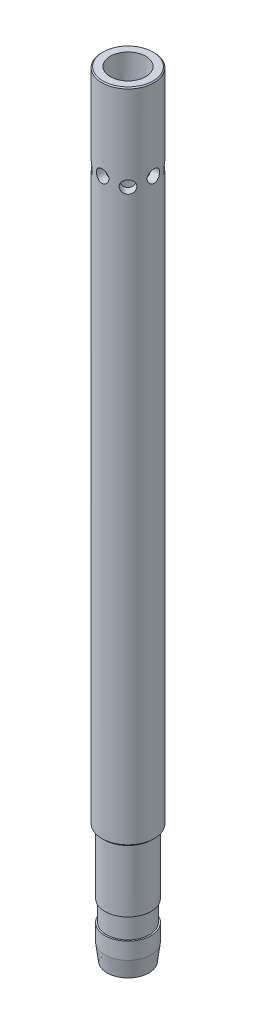
from build123d import *

# Parameters (mm, degrees)
SKETCH1_R           = 12.5
SKETCH1_R_2         = 8.5
BOSS_EXTRUDE1_DEPTH = 371
SKETCH2_R           = 16
SKETCH2_R_2         = 11
CUT_EXTRUDE1_DEPTH  = 56
SKETCH3_W           = 0.7
SKETCH3_H           = 10
CHAMFER1_SIZE       = 8
CHAMFER1_SIZE2      = 1
CHAMFER2_SIZE       = 1
SKETCH7_R           = 3
CUT_EXTRUDE4_DEPTH  = 24
CIRPATTERN2_COUNT   = 4
CHAMFER3_SIZE       = 0.5
SKETCH9_R           = 3
CUT_EXTRUDE11_DEPTH = 372.420920358
CIRPATTERN3_COUNT   = 4


with BuildPart() as part:
    # Sketch1 → Boss-Extrude1 (new body)
    with BuildSketch(Plane(origin=(0, 0, 0), x_dir=(1, 0, 0), z_dir=(0, 1, 0))):
        with Locations(Location((0, 0, 0), (0, 0, 270))):
            Circle(SKETCH1_R)
        with Locations(Location((0, 0, 0), (0, 0, 270))):
            Circle(SKETCH1_R_2, mode=Mode.SUBTRACT)
    extrude(amount=BOSS_EXTRUDE1_DEPTH)

    # Sketch2 → Cut-Extrude1 (cut)
    with BuildSketch(Plane.XZ):
        Circle(SKETCH2_R)
        with Locations(Location((0, 0, 0), (0, 0, 270))):
            Circle(SKETCH2_R_2, mode=Mode.SUBTRACT)
    extrude(amount=-CUT_EXTRUDE1_DEPTH, mode=Mode.SUBTRACT)

    # Sketch3 → Cut-Revolve1 (revolve, cut)
    with BuildSketch(Plane.XY, mode=Mode.PRIVATE) as cut_revolve1_sk:
        with Locations((10.65, 21)):
            Rectangle(SKETCH3_W, SKETCH3_H)
    revolve(cut_revolve1_sk.sketch.rotate(Axis((0, 357.5, 0), (0, -1, 0)), 270), axis=Axis((0, 357.5, 0), (0, -1, 0)), mode=Mode.SUBTRACT)

    # Chamfer1
    chamfer1_edges = [part.edges().sort_by_distance(p)[0] for p in [
        (0, 0, 11),
    ]]
    chamfer1_side = [part.faces().sort_by_distance(p)[0] for p in [
        (0, 8, 11),
    ]]
    chamfer(chamfer1_edges, length=CHAMFER1_SIZE, length2=CHAMFER1_SIZE2, reference=chamfer1_side[0])

    # Chamfer2
    chamfer2_edges = [part.edges().sort_by_distance(p)[0] for p in [
        (0, 56, -12.5),
    ]]
    chamfer(chamfer2_edges, length=CHAMFER2_SIZE)

    # Sketch7 → Cut-Extrude4 (cut)
    with BuildSketch(Plane.XY):
        with Locations(Location((0, 331.8, 0), (0, 0, 90))):
            Circle(SKETCH7_R)
    cut_extrude4 = extrude(amount=-CUT_EXTRUDE4_DEPTH, mode=Mode.SUBTRACT)

    # CirPattern2: Cut-Extrude4 ×4 about axis
    cirpattern2_axis = Axis((0, 371, 0), (0, -1, 0))
    for i in range(1, CIRPATTERN2_COUNT):
        add(cut_extrude4.rotate(cirpattern2_axis, i * 360 / CIRPATTERN2_COUNT), mode=Mode.SUBTRACT)

    # Chamfer3
    chamfer3_edges = [part.edges().sort_by_distance(p)[0] for p in [
        (0, 371, -12.5),
    ]]
    chamfer(chamfer3_edges, length=CHAMFER3_SIZE)

    # Sketch9 → Cut-Extrude11 (cut, through all)
    with BuildSketch(Plane(origin=(0, 0, 0), x_dir=(0.7071067811865464, 0, 0.7071067811865488), z_dir=(-0.7071067811865488, 0, 0.7071067811865464))):
        with Locations((0, 329.8)):
            Circle(SKETCH9_R)
    cut_extrude11 = extrude(amount=-CUT_EXTRUDE11_DEPTH, mode=Mode.SUBTRACT)

    # CirPattern3: Cut-Extrude11 ×4 about axis
    cirpattern3_axis = Axis((0, 371, 0), (0, -1, 0))
    for i in range(1, CIRPATTERN3_COUNT):
        add(cut_extrude11.rotate(cirpattern3_axis, i * 360 / CIRPATTERN3_COUNT), mode=Mode.SUBTRACT)


solid = part.part
